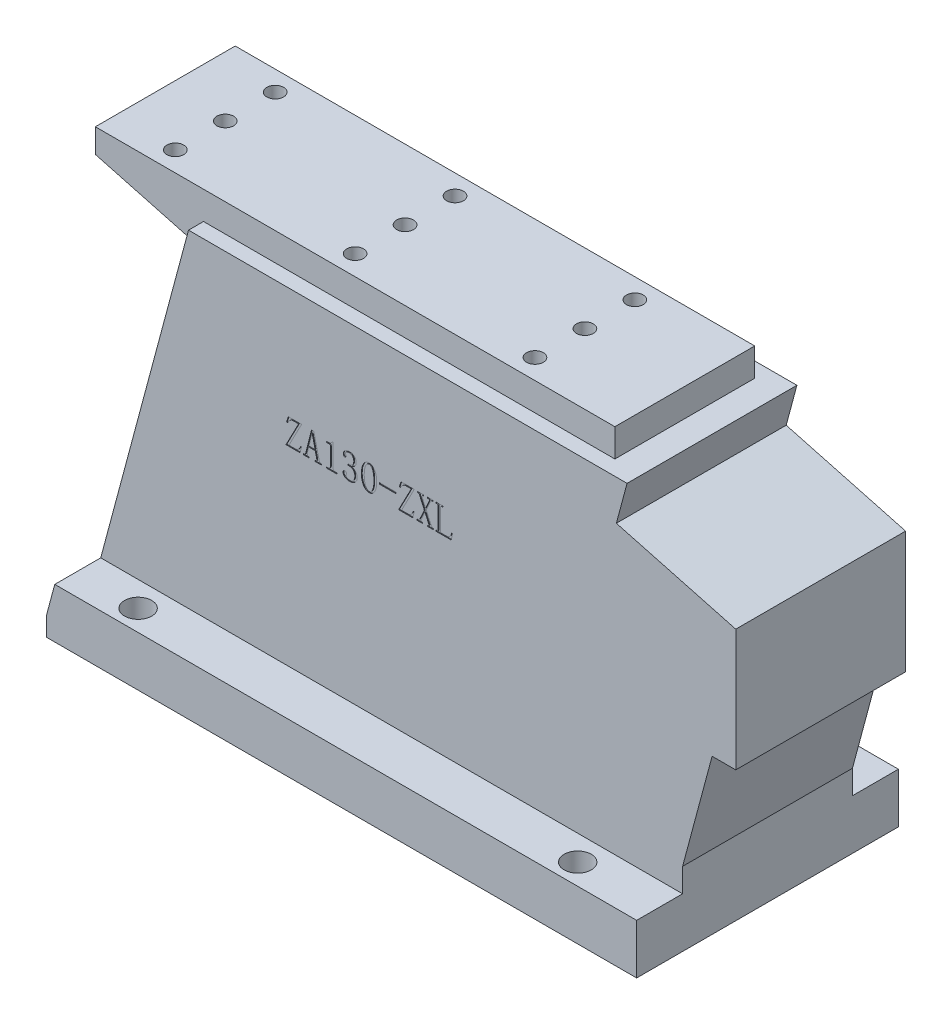
SolidWorks part; units mm, degrees
ref_plane "Front Plane" through (0, 0, 0) normal (0, 0, 1) x (1, 0, 0)
ref_plane "Top Plane" through (0, 0, 0) normal (0, 1, 0) x (1, 0, 0)
ref_plane "Right Plane" through (0, 0, 0) normal (1, 0, 0) x (0, 0, -1)
sketch "Sketch1" plane through (0, 0, 0) normal (0, 0, 1) x (1, 0, 0)
  line L0 (0, 0) -> (-130, 0)
  line L1 (-130, 0) -> (-130, -6)
  line L2 (-130, -6) -> (-104.5, -12.8327)
  line L3 (-104.5, -12.8327) -> (-104.5, 0) construction
  line L4 (0, 0) -> (0, -7)
  line L5 (0, -7) -> (6.8021, -7)
  line L6 (6.8021, -7) -> (4.1241, -16.9948)
  line L7 (4.1241, -16.9948) -> (34, -25)
  line L8 (34, -25) -> (34, -55.5)
  line L9 (34, -55.5) -> (28.0828, -55.5)
  line L10 (28.0828, -55.5) -> (20.7, -83.0529)
  line L11 (20.7, -83.0529) -> (20.7, -101.5)
  line L12 (20.7, -101.5) -> (-127, -101.5)
  line L13 (-127, -101.5) -> (-127, -96.8038)
  line L14 (-127, -96.8038) -> (-104.5, -12.8327)
  point P12 (5.4631, -11.9974)
  point P21 (31.0414, -55.5)
  point P23 (3.4011, -7)
  dimension "D1" = 15
  dimension "D2" = 6
  dimension "D3" = 25.5
  dimension "D4" = 75
  dimension "D5" = 130
  dimension "D6" = 106
  dimension "D7" = 101.5
  dimension "D8" = 3
  dimension "D9" = 147.7
  dimension "D10" = 164
  dimension "D11" = 25
  dimension "D12" = 46
  dimension "D13" = 7
extrude "Boss-Extrude1" add sketch "Sketch1" along normal mid plane 42.5
sketch "Sketch2" plane through (0, 0, 0) normal (0, 1, 0) x (1, 0, 0)
  line L0 (0, 0) -> (-145.8801, 0) construction
  line L1 (0, -21.25) -> (0, 21.25) construction
  line L2 (-130, 21.25) -> (0, 21.25)
  line L3 (-130, 21.25) -> (-130, 17.5)
  line L4 (-130, 17.5) -> (0, 17.5)
  line L5 (0, 21.25) -> (0, 17.5)
  line L6 (0, -21.25) -> (0, -17.5)
  line L7 (-130, -17.5) -> (0, -17.5)
  line L8 (-130, -21.25) -> (-130, -17.5)
  line L9 (-130, -21.25) -> (0, -21.25)
  dimension "D1" = 35
extrude "Cut-Extrude1" cut sketch "Sketch2" against normal blind 7
sketch "Sketch3" plane through (0, 0, 21.25) normal (0, 0, 1) x (1, 0, 0)
  line L0 (-104.5, -12.8327) -> (-102.9371, -7)
  line L1 (6.8021, -7) -> (-126.2679, -7) construction
  line L2 (-102.9371, -7) -> (-126.2679, -7)
  line L3 (-126.2679, -7) -> (-104.5, -12.8327)
extrude "Cut-Extrude2" cut sketch "Sketch3" against normal up to surface (3.75 mm away) up to face at (-77.2536, -4, 17.5)
sketch "Sketch4" plane through (0, 0, -21.25) normal (0, 0, -1) x (-1, 0, 0)
  line L3 (102.9371, -7) -> (104.5, -12.8327)
  line L4 (126.2679, -7) -> (102.9371, -7)
  line L5 (104.5, -12.8327) -> (126.2679, -7)
  line L6 (102.9371, -7) -> (104.5, -12.8327)
  line L7 (126.2679, -7) -> (102.9371, -7)
  line L8 (104.5, -12.8327) -> (126.2679, -7)
  dimension "D1" = 0
extrude "Cut-Extrude3" cut sketch "Sketch4" against normal up to surface (3.75 mm away) up to face at (-77.2536, -4, -17.5)
sketch "Sketch5" plane through (0, 0, 0) normal (0, 0, 1) x (1, 0, 0)
  line L0 (20.7, -101.5) -> (20.7, -83.0529) construction
  line L1 (-127, -101.5) -> (20.7, -101.5) construction
  line L2 (-127, -96.8038) -> (-127, -101.5) construction
  line L3 (20.7, -101.5) -> (20.7, -89)
  line L4 (-127, -101.5) -> (20.7, -101.5)
  line L5 (-127, -96.8038) -> (-127, -101.5)
  line L6 (-127, -96.8038) -> (-124.909, -89)
  line L7 (-102.9371, -7) -> (-127, -96.8038) construction
  line L8 (-124.909, -89) -> (20.7, -89)
  dimension "D1" = 12.5
extrude "Boss-Extrude2" add sketch "Sketch5" along normal mid plane 65.5
hole_wizard "M8 Tapped Hole1" positions "Sketch6" profile "Sketch7" tap size "M8" standard "GB" end condition through all
sketch "Sketch6" plane through (0, -101.5, 0) normal (0, -1, 0) x (-1, 0, 0)
  line L0 (0, 0) -> (166.3819, 0) construction
  line L4 (109.3, -27.5) -> (-0.7, -27.5)
  line L5 (109.3, -27.5) -> (109.3, 27.5)
  line L6 (109.3, 27.5) -> (-0.7, 27.5)
  line L7 (-0.7, -27.5) -> (-0.7, 27.5)
  line L10 (-20.7, -32.75) -> (-20.7, 32.75) construction
  line L11 (127, -32.75) -> (127, 32.75) construction
  point P8 (109.3, -27.5)
  point P9 (-0.7, 27.5)
  point P192 (109.3, 27.5)
  point P193 (-0.7, -27.5)
  dimension "D1" = 20
  dimension "D2" = 55
  dimension "D3" = 110
  dimension "D4" = 17.7
sketch "Sketch7" plane through (0.7, -101.5, 27.5) normal (1, 0, 0) x (0, 0, -1)
  line L0 (0, 0) -> (0, 101.5)
  line L1 (0, 101.5) -> (3.4, 101.5)
  line L2 (3.4, 101.5) -> (3.4, 0)
  line L5 (3.4, 0) -> (0, 0)
  line L11 (0, -6.35) -> (0, 107.95) construction
  dimension "通孔螺纹孔钻头直径" = 6.8
  dimension "通孔螺纹孔钻头深度" = 101.5
cosmetic thread "Cosmetic thread 1" parameters "D2"=8
cosmetic thread "Cosmetic thread 2" parameters "D2"=8
cosmetic thread "Cosmetic thread 3" parameters "D2"=8
cosmetic thread "Cosmetic thread 4" parameters "D2"=8
hole_wizard "M5 Tapped Hole1" positions "Sketch8" profile "Sketch9" tap size "M5" standard "GB"
sketch "Sketch8" plane through (0, 0, 0) normal (0, 1, 0) x (1, 0, 0)
  line L0 (0, 0) -> (-157.8764, 0) construction
  line L3 (-115, 46.1724) -> (-115, -41.4857) construction
  line L4 (-115, 0) -> (-70, 0) construction
  line L5 (-130, -17.5) -> (-130, 17.5) construction
  line L6 (0, -17.5) -> (0, 17.5) construction
  point P12 (-115, 12.5)
  point P15 (-115, -12.5)
  point P16 (-115, 0)
  point P21 (-70, 12.5)
  point P22 (-70, -12.5)
  point P23 (-70, 0)
  point P24 (-25, 12.5)
  point P25 (-25, -12.5)
  point P26 (-25, 0)
  dimension "D2" = 45
  dimension "D3" = 25
  dimension "D4" = 15
  dimension "D5" = 25
  dimension "D1" = 3
sketch "Sketch9" plane through (-25, 0, 0) normal (1, 0, 0) x (0, 0, 1)
  line L0 (0, 0) -> (0, 13.6618)
  line L1 (0, 13.6618) -> (2.1, 12.4)
  line L2 (2.1, 12.4) -> (2.1, 0)
  line L5 (2.1, 0) -> (0, 0)
  line L10 (0, 13.6618) -> (-2.1, 12.4) construction
  line L11 (0, -6.35) -> (0, 107.95) construction
  dimension "螺纹孔钻头直径" = 4.2
  dimension "螺纹孔钻头深度" = 12.4
  dimension "导头角度" = 118
cosmetic thread "Cosmetic thread 5" parameters "D1"=10, "D2"=5
cosmetic thread "Cosmetic thread 6" parameters "D1"=10, "D2"=5
cosmetic thread "Cosmetic thread 7" parameters "D1"=10, "D2"=5
cosmetic thread "Cosmetic thread 8" parameters "D1"=10, "D2"=5
cosmetic thread "Cosmetic thread 9" parameters "D1"=10, "D2"=5
cosmetic thread "Cosmetic thread 10" parameters "D1"=10, "D2"=5
cosmetic thread "Cosmetic thread 11" parameters "D1"=10, "D2"=5
cosmetic thread "Cosmetic thread 12" parameters "D1"=10, "D2"=5
cosmetic thread "Cosmetic thread 13" parameters "D1"=10, "D2"=5
sketch "Sketch10" plane through (0, 0, 21.25) normal (0, 0, 1) x (1, 0, 0)
  text T0 "ZA130-ZXL\r\n   "
extrude "Cut-Extrude4" cut sketch "Sketch10" against normal blind 0.2
sketch "Sketch11" plane through (0, 0, -21.25) normal (0, 0, -1) x (-1, 0, 0)
  line L0 (53.15, -101.5) -> (53.15, -37.5023) construction
  line L1 (127, -101.5) -> (-20.7, -101.5) construction
  circle A0 centre (53.15, -65.5) radius 3
  dimension "D1" = 36
  dimension "D2" = 6
extrude "Outlet position" add sketch "Sketch11" along normal blind 12
